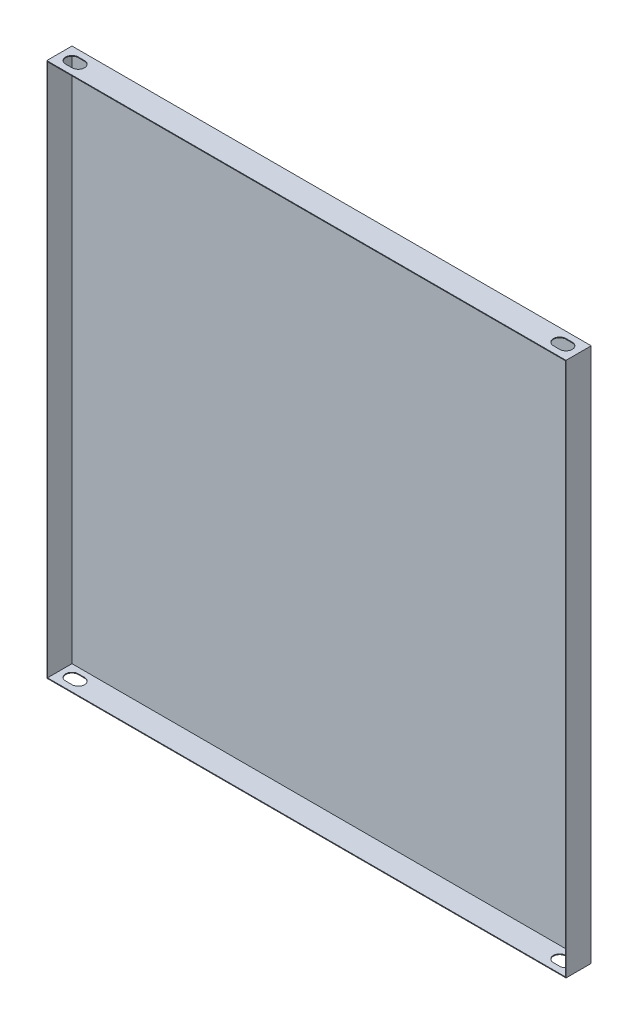
from build123d import *

# Parameters (mm, degrees)
SKETCH1_W           = 1650
SKETCH1_H           = 1700
BOSS_EXTRUDE1_DEPTH = 80
SHELL1_T            = -2.3
CUT_EXTRUDE1_DEPTH  = 1892.302461268


with BuildPart() as part:
    # Sketch1 → Boss-Extrude1 (new body)
    with BuildSketch(Plane.XY):
        Rectangle(SKETCH1_W, SKETCH1_H)
    extrude(amount=BOSS_EXTRUDE1_DEPTH)

    # Shell1
    shell1_openings = [part.faces().sort_by_distance(p)[0] for p in [
        (0, 0, 80),
    ]]
    offset(amount=SHELL1_T, openings=shell1_openings, kind=Kind.INTERSECTION)

    # Sketch2 → Cut-Extrude1 (cut, through all)
    with BuildSketch(Plane.XZ.offset(850)):
        with BuildLine():
            Line((-785, 60), (-765, 60))
            ThreePointArc((-765, 60), (-745, 40), (-765, 20))
            Line((-765, 20), (-785, 20))
            ThreePointArc((-785, 20), (-805, 40), (-785, 60))
        make_face()
        with BuildLine():
            Line((785, 60), (765, 60))
            ThreePointArc((765, 60), (745, 40), (765, 20))
            Line((765, 20), (785, 20))
            ThreePointArc((785, 20), (805, 40), (785, 60))
        make_face()
    extrude(amount=-CUT_EXTRUDE1_DEPTH, mode=Mode.SUBTRACT)


solid = part.part
